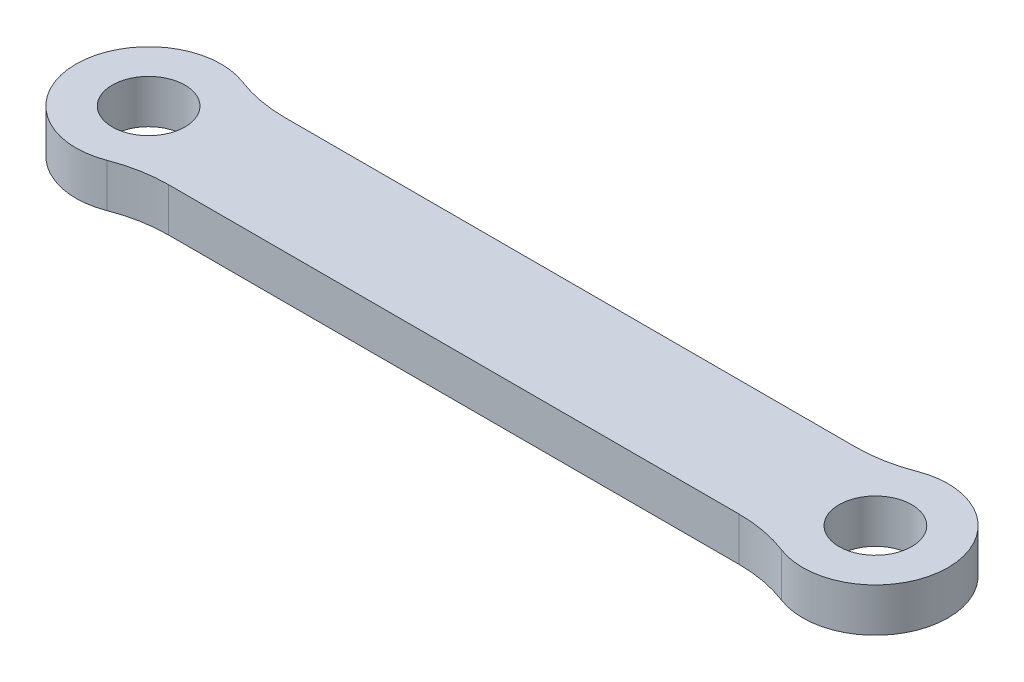
SolidWorks part; units mm, degrees
material "哈碳纤"
ref_plane "前视基准面" through (0, 0, 0) normal (0, 0, 1) x (1, 0, 0)
ref_plane "上视基准面" through (0, 0, 0) normal (0, 1, 0) x (1, 0, 0)
ref_plane "右视基准面" through (0, 0, 0) normal (1, 0, 0) x (0, 0, -1)
other "Configuration Table"
sketch "草图1" plane through (0, 0, 0) normal (0, 1, 0) x (1, 0, 0)
  line L0 (0, 0) -> (50, 0) construction
  line L1 (3, -4) -> (47, -4)
  line L2 (3, 4) -> (47, 4)
  line L3 (0, 4) -> (50, 4) construction
  line L4 (0, -4) -> (50, -4) construction
  arc A0 (47, -4) -> (47, 4) centre (50, 0) ccw
  arc A1 (3, 4) -> (3, -4) centre (0, 0) ccw
  circle A2 centre (0, 0) radius 2.5
  circle A3 centre (50, 0) radius 2.5
  dimension "D2" = 10
  dimension "D3" = 10
  dimension "D6" = 5
  dimension "D7" = 5
  dimension "D1" = 50
  dimension "D4" = 4
  dimension "D5" = 4
extrude "凸台-拉伸1" add sketch "草图1" along normal blind 3
fillet "圆角1" radius 10 4 edges at (3, 1.5, -4) (47, 1.5, -4) (47, 1.5, 4) (3, 1.5, 4)
